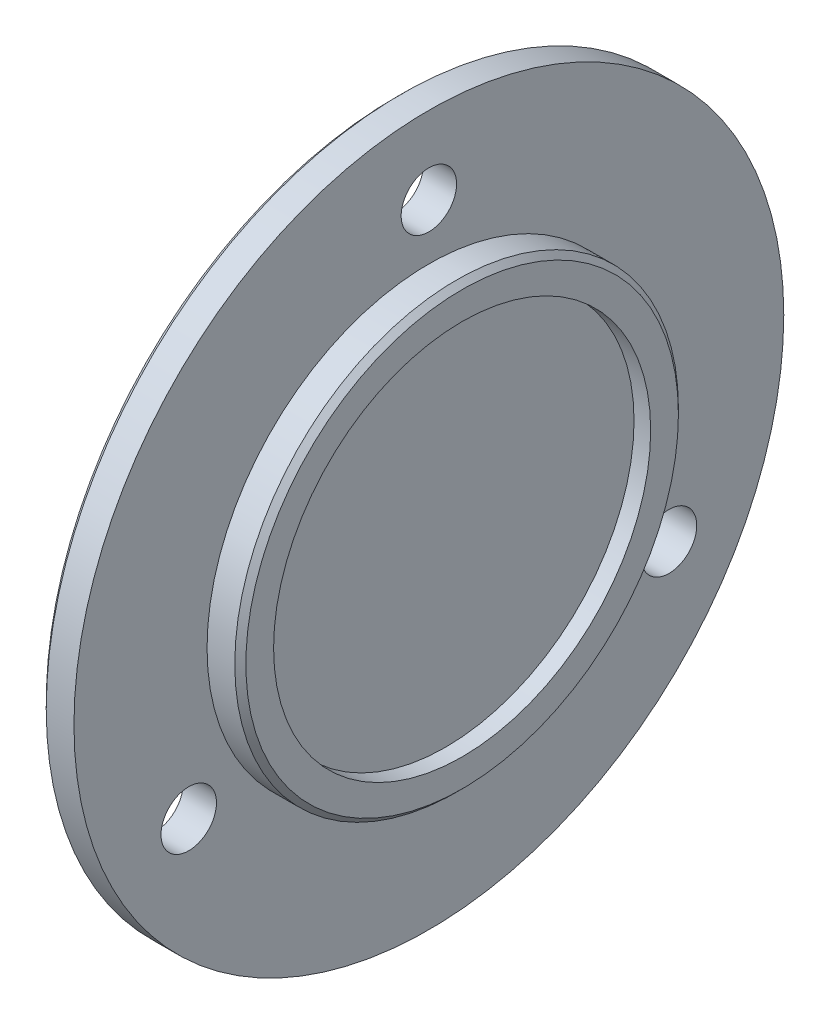
SolidWorks part; units mm, degrees
ref_plane "Front Plane" through (0, 0, 0) normal (0, 0, 1) x (1, 0, 0)
ref_plane "Top Plane" through (0, 0, 0) normal (0, 1, 0) x (1, 0, 0)
ref_plane "Right Plane" through (0, 0, 0) normal (1, 0, 0) x (0, 0, -1)
other "Configuration Table"
sketch "Sketch1" plane through (0, 0, 0) normal (1, 0, 0) x (0, 0, -1)
  circle A1 centre (0, 0) radius 32
  dimension "D1" = 64
extrude "Boss-Extrude1" add sketch "Sketch1" along normal blind 3
sketch "Sketch2" plane through (3, 0, 0) normal (1, 0, 0) x (0, 0, -1)
  circle A0 centre (0, 0) radius 20
  dimension "D1" = 40
extrude "Boss-Extrude2" add sketch "Sketch2" along normal blind 3
sketch "Sketch3" plane through (6, 0, 0) normal (1, 0, 0) x (0, 0, -1)
  circle A0 centre (0, 0) radius 17
  dimension "D1" = 34
extrude "Cut-Extrude1" cut sketch "Sketch3" against normal blind 1.5
sketch "Sketch4" plane through (0, 0, 0) normal (-1, 0, 0) x (0, 0, 1)
  line L0 (0, 25) -> (0, 0) construction
  circle A0 centre (0, 25) radius 2.5
  circle A1 centre (21.6506, -12.5) radius 2.5
  circle A2 centre (-21.6506, -12.5) radius 2.5
  point P11 (0, 0)
  dimension "D2" = 5
  dimension "D1" = 25
  dimension "D3" = 3
extrude "Cut-Extrude2" cut sketch "Sketch4" against normal blind 36.5
chamfer "Chamfer1" distance 0.5 angle 45 2 edges at (6, 0, -20) (0, 0, -32)
